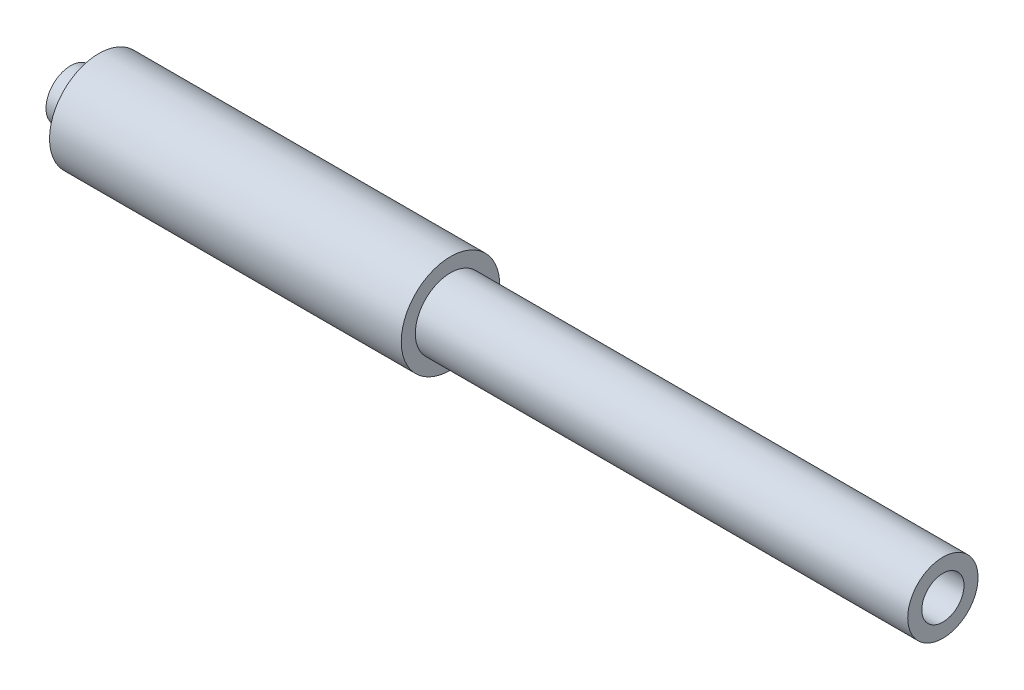
from build123d import *


with BuildPart() as part:
    # Sketch1 → Revolve1 (revolve)
    with BuildSketch(Plane.XY, mode=Mode.PRIVATE) as revolve1_sk:
        Polygon((631.173921275, 208.284534899), (631.173921275, 218.284534899), (281.173921275, 218.284534899), (281.173921275, 228.284534899), (31.173921275, 228.284534899), (31.173921275, 210.784534899), (11.173921275, 210.784534899), (11.173921275, 200.784534899), (41.173921275, 200.784534899), (41.173921275, 218.284534899), (271.173921275, 218.284534899), (271.173921275, 208.284534899), align=None)
    revolve(revolve1_sk.sketch.rotate(Axis((-12.5607058, 193.284534899, 0), (1, 0, 0)), 90), axis=Axis((-12.5607058, 193.284534899, 0), (1, 0, 0)))


solid = part.part
